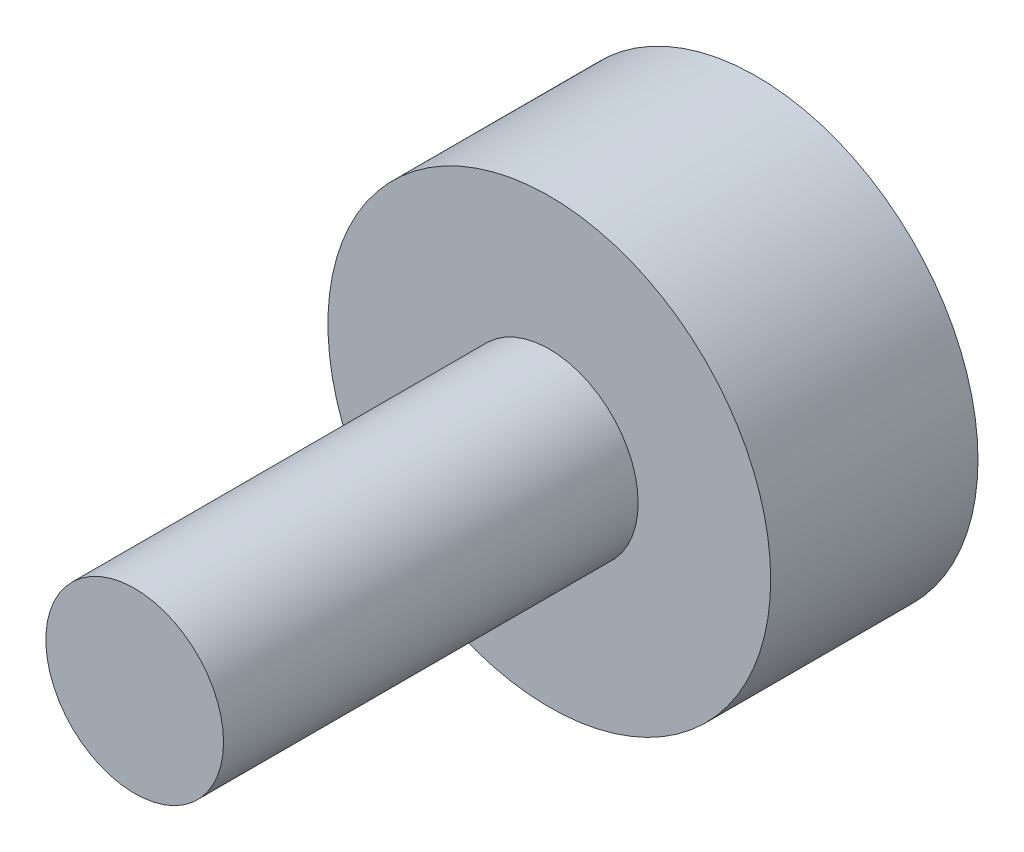
from build123d import *

# Parameters (mm, degrees)
SKETCH_1_R          = 74.75
EXTRUDE_1_DEPTH     = 70
SKETCH_2_R          = 16.25
CUT_EXTRUDE_1_DEPTH = 68
SKETCH_3_R          = 30
EXTRUDE_2_DEPTH     = 140


with BuildPart() as part:
    # 草图1 → 凸台-拉伸1 (new body)
    with BuildSketch(Plane.XY):
        Circle(SKETCH_1_R)
    extrude(amount=EXTRUDE_1_DEPTH)

    # 草图2 → 切除-拉伸1 (cut)
    with BuildSketch(Plane(origin=(0, 0, 0), x_dir=(-1, 0, 0), z_dir=(0, 0, -1))):
        Circle(SKETCH_2_R)
    extrude(amount=-CUT_EXTRUDE_1_DEPTH, mode=Mode.SUBTRACT)

    # 草图3 → 凸台-拉伸2 (add)
    with BuildSketch(Plane.XY.offset(70)):
        Circle(SKETCH_3_R)
    extrude(amount=EXTRUDE_2_DEPTH)


solid = part.part
